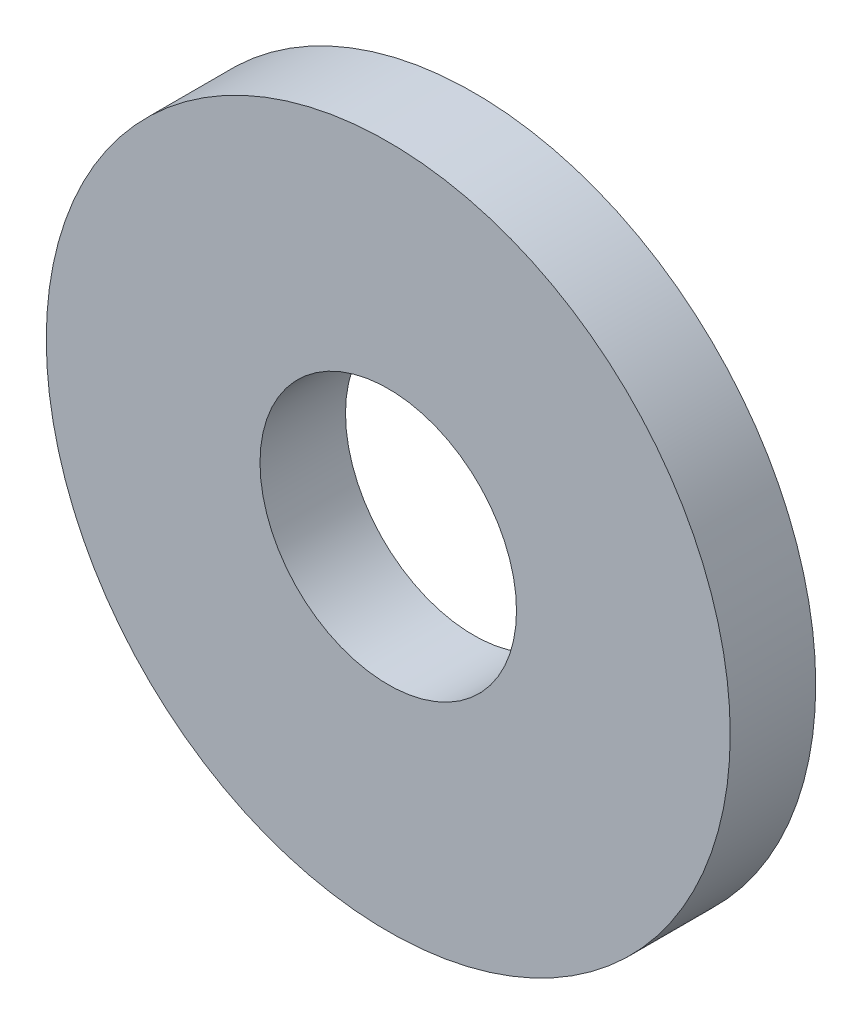
from build123d import *

# Parameters (mm, degrees)
SKETCH1_R           = 4
SKETCH1_R_2         = 1.5
BOSS_EXTRUDE1_DEPTH = 1


with BuildPart() as part:
    # Sketch1 → Boss-Extrude1 (new body)
    with BuildSketch(Plane.XY):
        Circle(SKETCH1_R)
        Circle(SKETCH1_R_2, mode=Mode.SUBTRACT)
    extrude(amount=BOSS_EXTRUDE1_DEPTH)


solid = part.part
